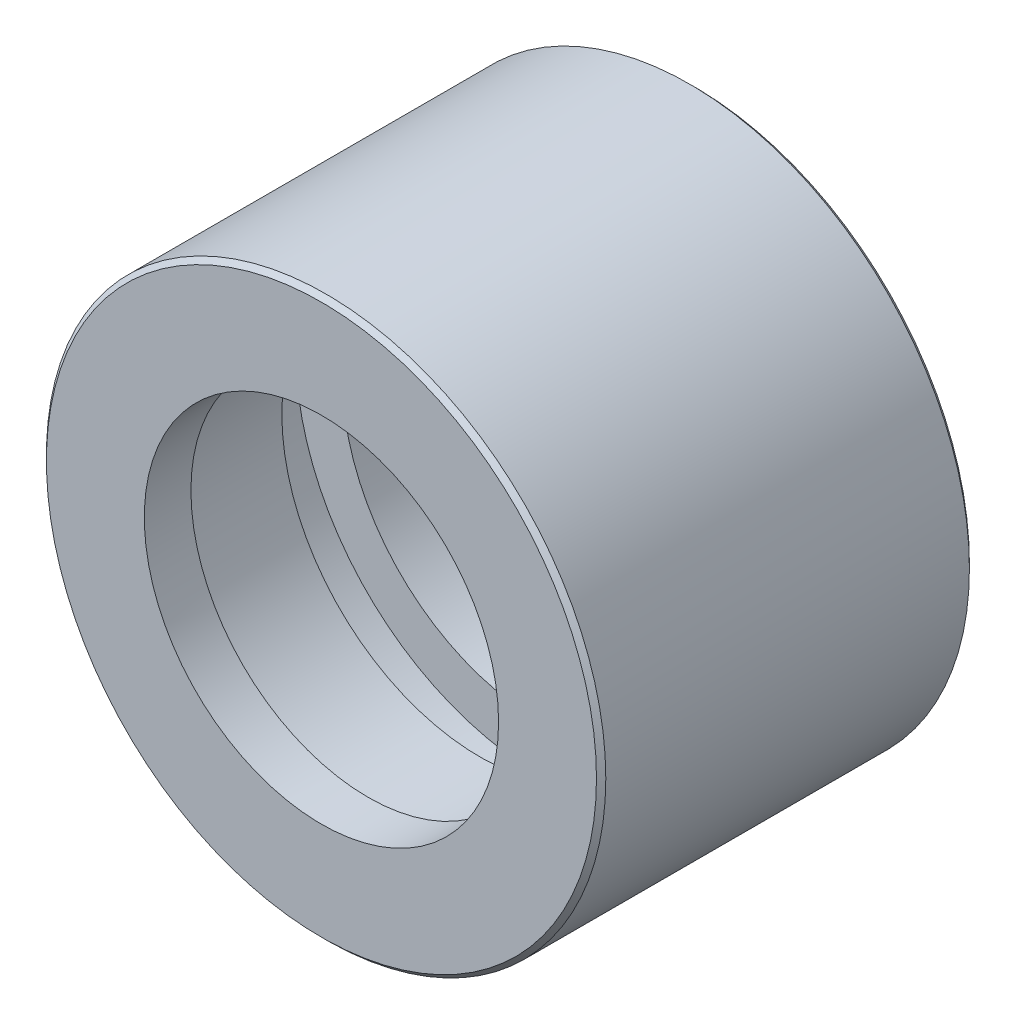
SolidWorks part; units mm, degrees
ref_plane "前视基准面" through (0, 0, 0) normal (0, 0, 1) x (1, 0, 0)
ref_plane "上视基准面" through (0, 0, 0) normal (0, 1, 0) x (1, 0, 0)
ref_plane "右视基准面" through (0, 0, 0) normal (1, 0, 0) x (0, 0, -1)
sketch "草图1" plane through (0, 0, 0) normal (0, 0, 1) x (1, 0, 0)
  circle A0 centre (0, 0) radius 60
  dimension "D1" = 120
extrude "凸台-拉伸1" add sketch "草图1" along normal blind 80
sketch "草图2" plane through (0, 0, 0) normal (0, 0, -1) x (-1, 0, 0)
  circle A0 centre (0, 0) radius 42.5
  dimension "D1" = 85
extrude "切除-拉伸1" cut sketch "草图2" against normal blind 70
sketch "草图3" plane through (0, 0, 80) normal (0, 0, 1) x (1, 0, 0)
  circle A0 centre (0, 0) radius 38
  dimension "D1" = 76
extrude "切除-拉伸2" cut sketch "草图3" against normal blind 70
chamfer "倒角1" distance 1 angle 45 2 edges at (60, 0, 0) (60, 0, 80)
ref_plane "基准面2" through (0, 0, 10) normal (0, 0, -1) x (-1, 0, 0)
sketch "草图4" plane through (0, 0, 10) normal (0, 0, -1) x (-1, 0, 0)
  circle A0 centre (0, 0) radius 52.5
  circle A1 centre (0, 0) radius 42.5
  dimension "D1" = 105
extrude "切除-拉伸3" cut sketch "草图4" against normal blind 13
ref_plane "基准面3" through (0, 0, 33) normal (0, 0, -1) x (-1, 0, 0)
sketch "草图5" plane through (0, 0, 33) normal (0, 0, -1) x (-1, 0, 0)
  circle A0 centre (0, 0) radius 52.5
  circle A1 centre (0, 0) radius 42.5
  dimension "D1" = 105
  dimension "D2" = 85
extrude "切除-拉伸4" cut sketch "草图5" against normal blind 13
